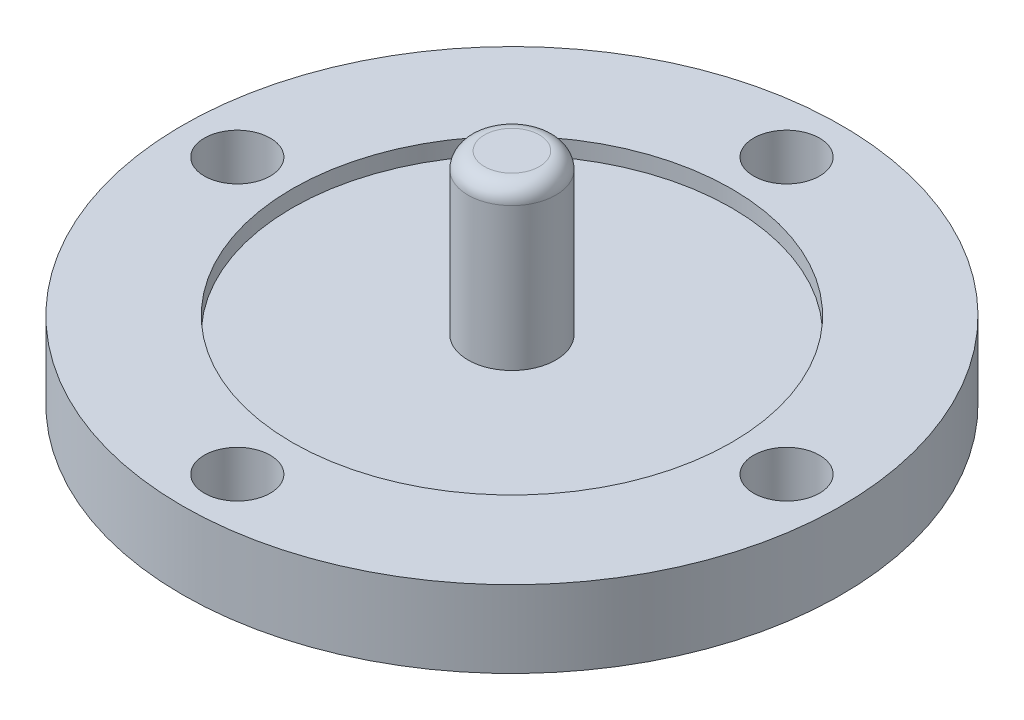
from build123d import *

# Parameters (mm, degrees)
SKETCH1_R           = 30
BOSS_EXTRUDE1_DEPTH = 7
SKETCH2_R           = 4
BOSS_EXTRUDE2_DEPTH = 13
CUT_EXTRUDE1_START  = -1.5
SKETCH3_R           = 20
SKETCH3_R_2         = 4
CUT_EXTRUDE1_DEPTH  = 1.5
HOLE1_D             = 6
HOLE1_CSINK_D       = 9
HOLE1_CSINK_ANGLE   = 90
FILLET1_R           = 1.5


with BuildPart() as part:
    # Sketch1 → Boss-Extrude1 (new body)
    with BuildSketch(Plane(origin=(0, 0, 0), x_dir=(1, 0, 0), z_dir=(0, 1, 0))):
        with Locations(Location((0, 0, 0), (0, 0, 270))):
            Circle(SKETCH1_R)
    extrude(amount=BOSS_EXTRUDE1_DEPTH)

    # Sketch2 → Boss-Extrude2 (add)
    with BuildSketch(Plane(origin=(0, 7, 0), x_dir=(1, 0, 0), z_dir=(0, 1, 0))):
        with Locations(Location((0, 0, 0), (0, 0, 90))):
            Circle(SKETCH2_R)
    extrude(amount=BOSS_EXTRUDE2_DEPTH)

    # Sketch3 → Cut-Extrude1 (cut)
    with BuildSketch(Plane(origin=(0, 7, 0), x_dir=(1, 0, 0), z_dir=(0, 1, 0)).offset(CUT_EXTRUDE1_START)):
        with Locations(Location((0, 0, 0), (0, 0, 270))):
            Circle(SKETCH3_R)
        with Locations(Location((0, 0, 0), (0, 0, 90))):
            Circle(SKETCH3_R_2, mode=Mode.SUBTRACT)
    extrude(amount=CUT_EXTRUDE1_DEPTH, mode=Mode.SUBTRACT)

    # Hole1 (through all)
    with Locations(Plane(origin=(0, 0, 0), x_dir=(-1, 0, 0), z_dir=(0, -1, 0))):
        with Locations((-25, 0), (0, 25), (25, 0), (0, -25)):
            CounterSinkHole(HOLE1_D / 2, HOLE1_CSINK_D / 2, counter_sink_angle=HOLE1_CSINK_ANGLE)

    # Fillet1
    fillet1_edges = [part.edges().sort_by_distance(p)[0] for p in [
        (0, 20, 4),
    ]]
    fillet(fillet1_edges, radius=FILLET1_R)


solid = part.part
